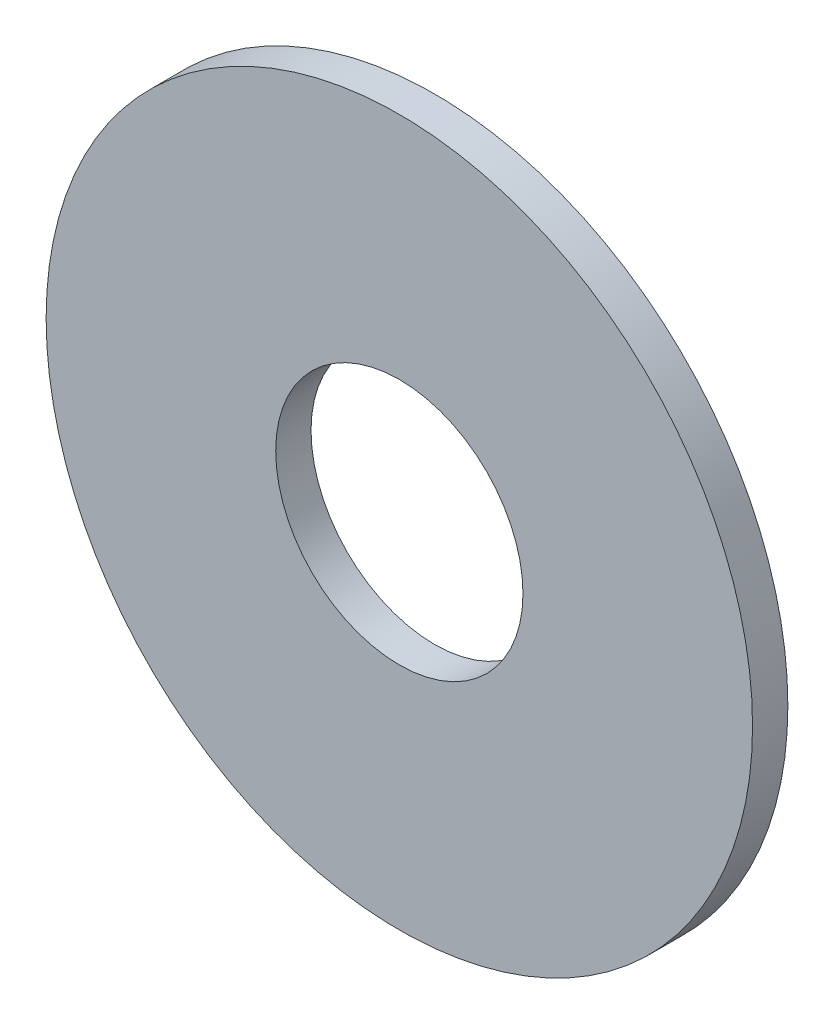
SolidWorks part; units mm, degrees
ref_plane "Front Plane" through (0, 0, 0) normal (0, 0, 1) x (1, 0, 0)
ref_plane "Top Plane" through (0, 0, 0) normal (0, 1, 0) x (1, 0, 0)
ref_plane "Right Plane" through (0, 0, 0) normal (1, 0, 0) x (0, 0, -1)
sketch "Sketch1" plane through (0, 0, 0) normal (0, 0, 1) x (1, 0, 0)
  circle A0 centre (0, 0) radius 10
  circle A1 centre (0, 0) radius 3.5
  dimension "D1" = 7
  dimension "D2" = 20
extrude "Boss-Extrude1" add sketch "Sketch1" along normal blind 1
